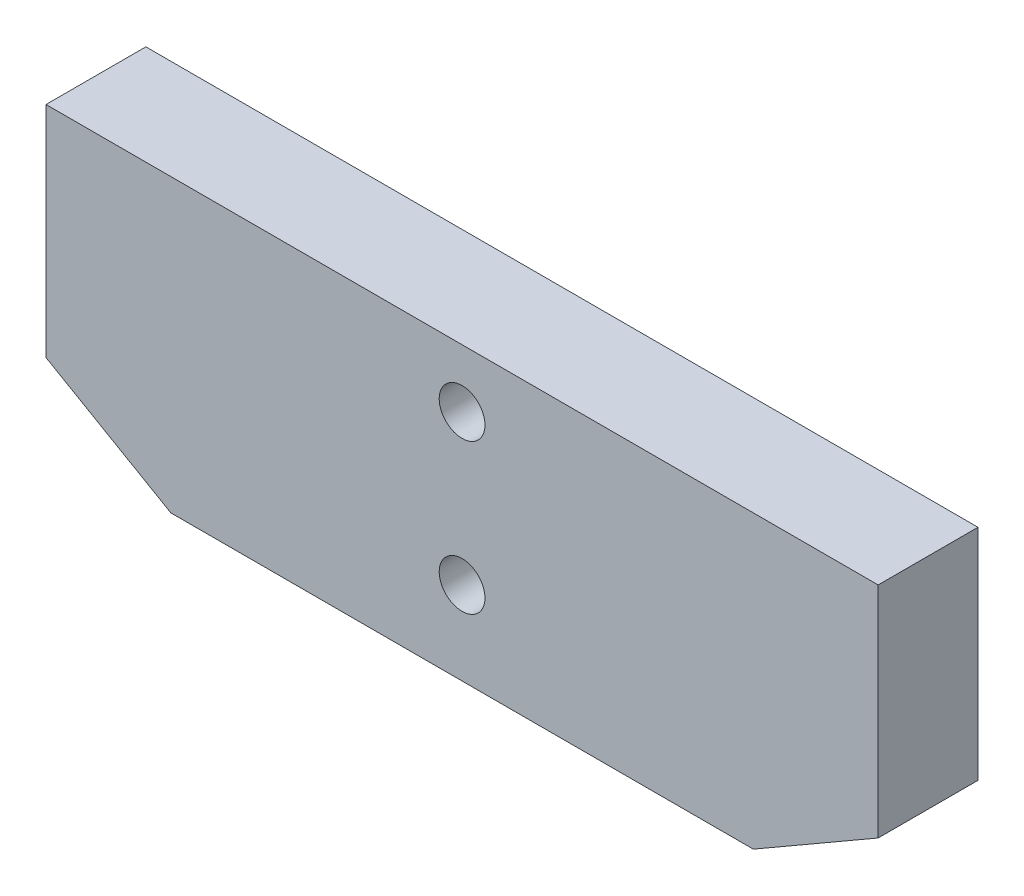
from build123d import *

# Parameters (mm, degrees)
SKETCH_1_W                = 100
SKETCH_1_H                = 35
EXTRUDE_1_DEPTH           = 12
CHAMFER_1_SIZE            = 15
CHAMFER_1_SIZE2           = 8.660254038
HOLE_WIZARD_1_D           = 5.5
HOLE_WIZARD_1_CBORE_D     = 10
HOLE_WIZARD_1_CBORE_DEPTH = 5.7


with BuildPart() as part:
    # 草图1 → 凸台-拉伸1 (new body)
    with BuildSketch(Plane.XY):
        Rectangle(SKETCH_1_W, SKETCH_1_H)
    extrude(amount=EXTRUDE_1_DEPTH)

    # 倒角1
    chamfer_1_edges = [part.edges().sort_by_distance(p)[0] for p in [
        (50, -17.5, 6),
        (-50, -17.5, 6),
    ]]
    chamfer_1_side = [part.faces().sort_by_distance(p)[0] for p in [
        (0, -17.5, 6),
    ]]
    chamfer(chamfer_1_edges, length=CHAMFER_1_SIZE, length2=CHAMFER_1_SIZE2, reference=chamfer_1_side[0])

    # 打孔尺寸(%根据)内六角圆柱头螺钉的类型1 (through all)
    with Locations(Plane(origin=(0, 0, 0), x_dir=(-1, 0, 0), z_dir=(0, 0, -1))):
        with Locations((0, 10.5), (0, -7.5)):
            CounterBoreHole(HOLE_WIZARD_1_D / 2, HOLE_WIZARD_1_CBORE_D / 2, HOLE_WIZARD_1_CBORE_DEPTH)


solid = part.part
